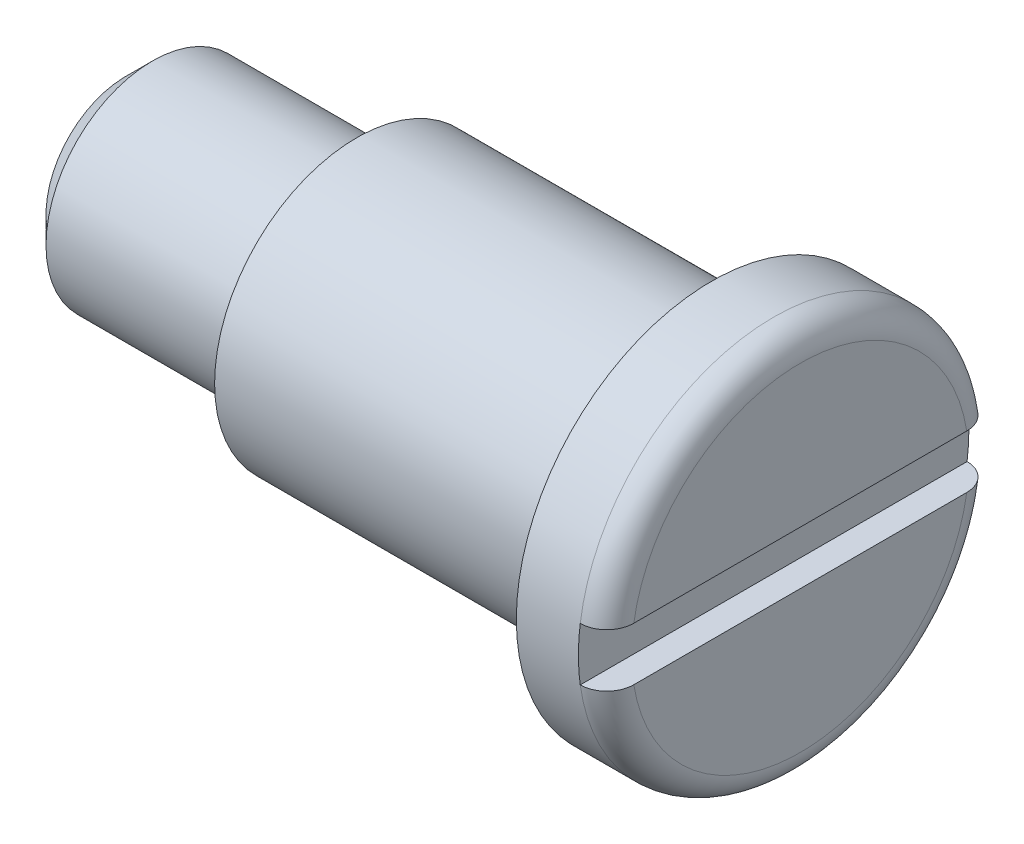
from build123d import *

# Parameters (mm, degrees)
SKETCH2_W          = 26.278844289
SKETCH2_H          = 3
CUT_EXTRUDE1_DEPTH = 1.5
FILLET1_R          = 1.5
CHAMFER1_SIZE      = 1.5


with BuildPart() as part:
    # Sketch1 → Revolve1 (revolve)
    with BuildSketch(Plane(origin=(0, 0, 0), x_dir=(1, 0, 0), z_dir=(0, 1, 0)), mode=Mode.PRIVATE) as revolve1_sk:
        Polygon((-19, 0), (-19, 6), (-6, 6), (-6, 8), (14, 8), (14, 11), (19, 11), (19, 0), align=None)
    revolve(revolve1_sk.sketch.rotate(Axis((-19, 0, 0), (1, 0, 0)), 180), axis=Axis((-19, 0, 0), (1, 0, 0)))

    # Sketch2 → Cut-Extrude1 (cut)
    with BuildSketch(Plane(origin=(19, 0, 0), x_dir=(0, 0, -1), z_dir=(1, 0, 0))):
        with Locations((0.853209231, 0)):
            Rectangle(SKETCH2_W, SKETCH2_H)
    extrude(amount=-CUT_EXTRUDE1_DEPTH, mode=Mode.SUBTRACT)

    # Fillet1
    fillet1_edges = [part.edges().sort_by_distance(p)[0] for p in [
        (19, -11, 0),
        (19, 11, 0),
    ]]
    fillet(fillet1_edges, radius=FILLET1_R)

    # Chamfer1
    chamfer1_edges = [part.edges().sort_by_distance(p)[0] for p in [
        (-19, 0, -6),
    ]]
    chamfer(chamfer1_edges, length=CHAMFER1_SIZE)


solid = part.part
